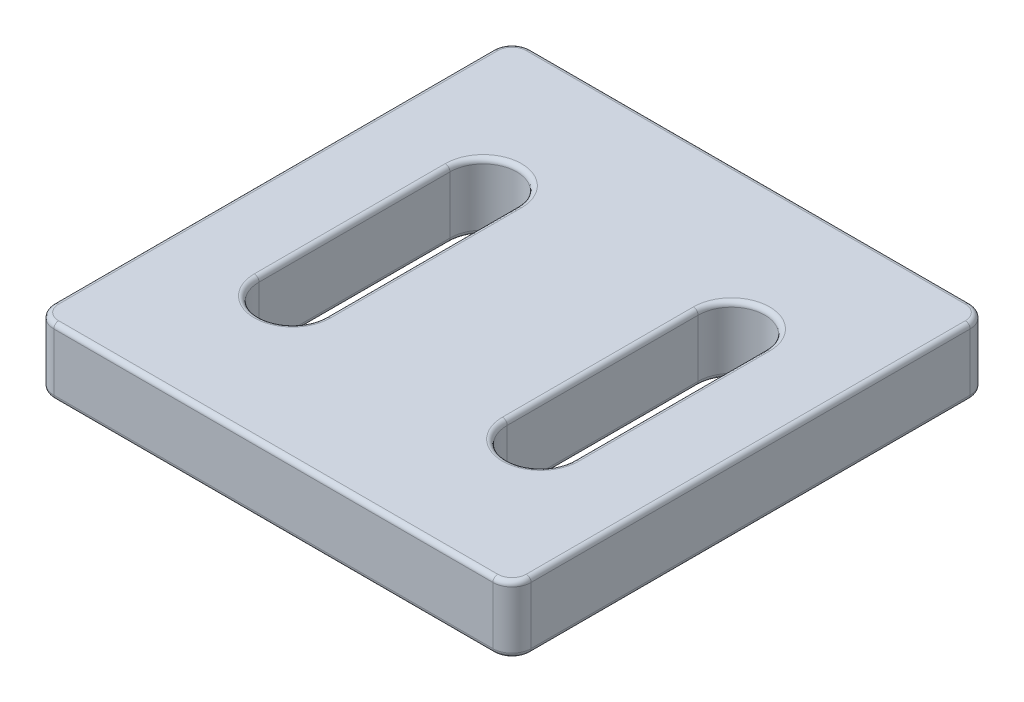
from build123d import *

# Parameters (mm, degrees)
BOSS_EXTRUDE1_DEPTH = 3.5
FILLET1_R           = 0.25


with BuildPart() as part:
    # Sketch1 → Boss-Extrude1 (new body)
    with BuildSketch(Plane(origin=(0, 0, 0), x_dir=(1, 0, 0), z_dir=(0, 1, 0))):
        with BuildLine():
            Line((-11.5, 12.5), (11.5, 12.5))
            ThreePointArc((11.5, 12.5), (12.207106781, 12.207106781), (12.5, 11.5))
            Line((12.5, 11.5), (12.5, -11.5))
            ThreePointArc((12.5, -11.5), (12.207106781, -12.207106781), (11.5, -12.5))
            Line((11.5, -12.5), (-11.5, -12.5))
            ThreePointArc((-11.5, -12.5), (-12.207106781, -12.207106781), (-12.5, -11.5))
            Line((-12.5, -11.5), (-12.5, 11.5))
            ThreePointArc((-12.5, 11.5), (-12.207106781, 12.207106781), (-11.5, 12.5))
        make_face()
        with BuildLine():
            Line((-8.25, -5), (-8.25, 5))
            ThreePointArc((-8.25, 5), (-6.5, 6.75), (-4.75, 5))
            Line((-4.75, 5), (-4.75, -5))
            ThreePointArc((-4.75, -5), (-6.5, -6.75), (-8.25, -5))
        make_face(mode=Mode.SUBTRACT)
        with BuildLine():
            Line((8.25, -5), (8.25, 5))
            ThreePointArc((8.25, 5), (6.5, 6.75), (4.75, 5))
            Line((4.75, 5), (4.75, -5))
            ThreePointArc((4.75, -5), (6.5, -6.75), (8.25, -5))
        make_face(mode=Mode.SUBTRACT)
    extrude(amount=BOSS_EXTRUDE1_DEPTH)

    # Fillet1
    fillet1_edges = [part.edges().sort_by_distance(p)[0] for p in [
        (0, 0, 12.5),
        (-12.207106781, 0, 12.207106781),
        (-12.5, 0, 0),
        (-12.207106781, 0, -12.207106781),
        (-12.207106781, 3.5, 12.207106781),
        (0, 3.5, 12.5),
        (12.207106781, 3.5, 12.207106781),
        (-6.5, 0, 6.75),
        (-4.75, 0, 0),
        (12.5, 3.5, 0),
        (-6.5, 0, -6.75),
        (-8.25, 0, 0),
        (-6.5, 3.5, 6.75),
        (-4.75, 3.5, 0),
        (-6.5, 3.5, -6.75),
        (-8.25, 3.5, 0),
        (12.207106781, 3.5, -12.207106781),
        (0, 3.5, -12.5),
        (6.5, 0, 6.75),
        (8.25, 0, 0),
        (6.5, 0, -6.75),
        (4.75, 0, 0),
        (6.5, 3.5, 6.75),
        (8.25, 3.5, 0),
        (6.5, 3.5, -6.75),
        (4.75, 3.5, 0),
        (-12.207106781, 3.5, -12.207106781),
        (0, 0, -12.5),
        (-12.5, 3.5, 0),
        (12.207106781, 0, -12.207106781),
        (12.5, 0, 0),
        (12.207106781, 0, 12.207106781),
    ]]
    fillet(fillet1_edges, radius=FILLET1_R)


solid = part.part
